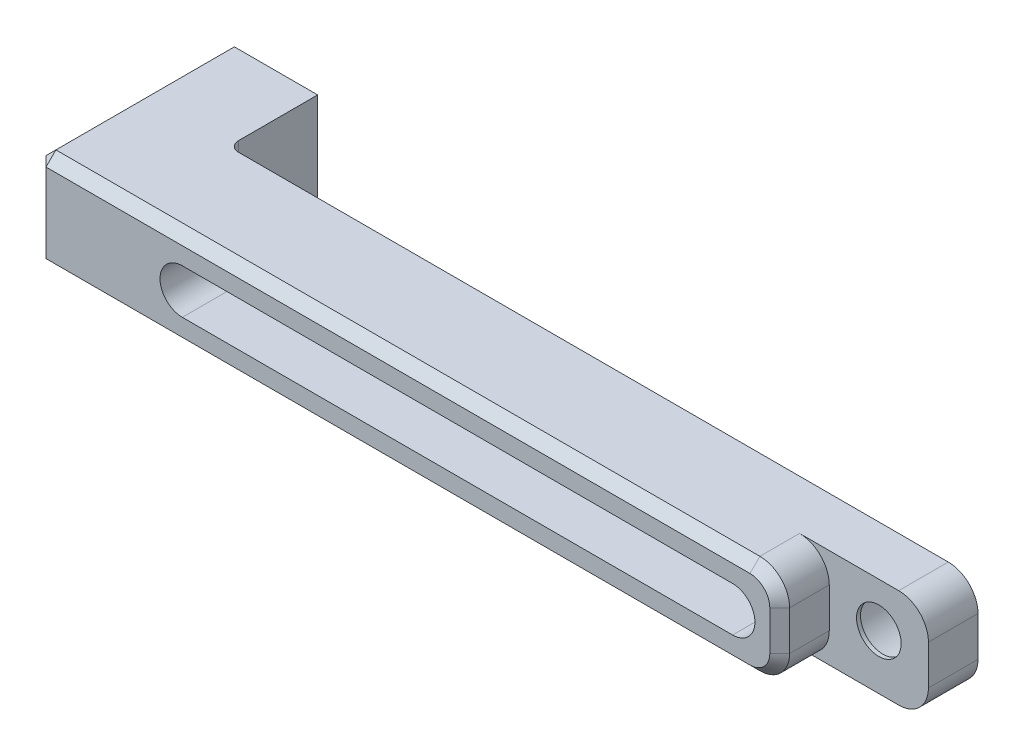
from build123d import *

# Parameters (mm, degrees)
SKETCH1_W                                            = 85
SKETCH1_H                                            = 10
BOSS_EXTRUDE1_DEPTH                                  = 10
CUT_EXTRUDE1_DEPTH                                   = 4.4
CUT_EXTRUDE2_DEPTH                                   = 45.018291652
SKETCH4_W                                            = 9.4
SKETCH4_H                                            = 10
BOSS_EXTRUDE2_DEPTH                                  = 10
SKETCH5_W                                            = 10
SKETCH5_H                                            = 10
CUT_EXTRUDE3_DEPTH                                   = 5
M6_TAPPED_HOLE1_D                                    = 5
M6_TAPPED_HOLE1_DEPTH                                = 5
M6_TAPPED_HOLE1_TIP                                  = 1.502151548
CBORE_FOR_M4_HEXAGON_SOCKET_HEAD_CAP_SCR_D           = 4.5
CBORE_FOR_M4_HEXAGON_SOCKET_HEAD_CAP_SCR_DEPTH       = 14
CBORE_FOR_M4_HEXAGON_SOCKET_HEAD_CAP_SCR_CBORE_D     = 8
CBORE_FOR_M4_HEXAGON_SOCKET_HEAD_CAP_SCR_CBORE_DEPTH = 4.6
CBORE_FOR_M4_HEXAGON_SOCKET_HEAD_CAP_SCR_TIP         = 1.351936393
FILLET1_R                                            = 3
FILLET2_R                                            = 1
CHAMFER1_SIZE                                        = 1


with BuildPart() as part:
    # Sketch1 → Boss-Extrude1 (new body)
    with BuildSketch(Plane(origin=(0, 0, 0), x_dir=(1, 0, 0), z_dir=(0, 1, 0))):
        Rectangle(SKETCH1_W, SKETCH1_H)
    extrude(amount=BOSS_EXTRUDE1_DEPTH)

    # Sketch2 → Cut-Extrude1 (cut)
    with BuildSketch(Plane.XY.offset(-5)):
        with BuildLine():
            Line((-27.75, 9), (27.75, 9))
            ThreePointArc((27.75, 9), (31.75, 5), (27.75, 1))
            Line((27.75, 1), (-27.75, 1))
            ThreePointArc((-27.75, 1), (-31.75, 5), (-27.75, 9))
        make_face()
    extrude(amount=CUT_EXTRUDE1_DEPTH, mode=Mode.SUBTRACT)

    # Sketch3 → Cut-Extrude2 (cut, through all)
    with BuildSketch(Plane(origin=(0, 0, -0.6), x_dir=(-1, 0, 0), z_dir=(0, 0, -1))):
        with BuildLine():
            Line((-27.75, 7.25), (27.75, 7.25))
            ThreePointArc((27.75, 7.25), (30, 5), (27.75, 2.75))
            Line((27.75, 2.75), (-27.75, 2.75))
            ThreePointArc((-27.75, 2.75), (-30, 5), (-27.75, 7.25))
        make_face()
    extrude(amount=-CUT_EXTRUDE2_DEPTH, mode=Mode.SUBTRACT)

    # Sketch4 → Boss-Extrude2 (add)
    with BuildSketch(Plane.XY.offset(-5)):
        with Locations((-37.8, 5)):
            Rectangle(SKETCH4_W, SKETCH4_H)
    extrude(amount=-BOSS_EXTRUDE2_DEPTH)

    # Sketch5 → Cut-Extrude3 (cut)
    with BuildSketch(Plane.XY.offset(5)):
        with Locations((37.5, 5)):
            Rectangle(SKETCH5_W, SKETCH5_H)
    extrude(amount=-CUT_EXTRUDE3_DEPTH, mode=Mode.SUBTRACT)

    # M6 Tapped Hole1
    with Locations(Plane(origin=(0, 0, -15), x_dir=(-1, 0, 0), z_dir=(0, 0, -1))):
        with Locations((37.8, 4.802472567)):
            Hole(M6_TAPPED_HOLE1_D / 2, depth=M6_TAPPED_HOLE1_DEPTH)
            with Locations((0, 0, -(M6_TAPPED_HOLE1_DEPTH + M6_TAPPED_HOLE1_TIP / 2))):  # 118° drill point
                Cone(0, M6_TAPPED_HOLE1_D / 2, M6_TAPPED_HOLE1_TIP, mode=Mode.SUBTRACT)

    # CBORE for M4 Hexagon socket head cap screws1
    with Locations(Plane(origin=(0, 0, -5), x_dir=(-1, 0, 0), z_dir=(0, 0, -1))):
        with Locations((-37.5, 5.5)):
            CounterBoreHole(CBORE_FOR_M4_HEXAGON_SOCKET_HEAD_CAP_SCR_D / 2, CBORE_FOR_M4_HEXAGON_SOCKET_HEAD_CAP_SCR_CBORE_D / 2, CBORE_FOR_M4_HEXAGON_SOCKET_HEAD_CAP_SCR_CBORE_DEPTH, depth=CBORE_FOR_M4_HEXAGON_SOCKET_HEAD_CAP_SCR_DEPTH)
            with Locations((0, 0, -(CBORE_FOR_M4_HEXAGON_SOCKET_HEAD_CAP_SCR_DEPTH + CBORE_FOR_M4_HEXAGON_SOCKET_HEAD_CAP_SCR_TIP / 2))):  # 118° drill point
                Cone(0, CBORE_FOR_M4_HEXAGON_SOCKET_HEAD_CAP_SCR_D / 2, CBORE_FOR_M4_HEXAGON_SOCKET_HEAD_CAP_SCR_TIP, mode=Mode.SUBTRACT)

    # Fillet1
    fillet1_edges = [part.edges().sort_by_distance(p)[0] for p in [
        (42.5, 0, -2.5),
        (42.5, 10, -2.5),
        (32.5, 0, 2.5),
        (32.5, 10, 2.5),
    ]]
    fillet(fillet1_edges, radius=FILLET1_R)

    # Fillet2
    fillet2_edges = [part.edges().sort_by_distance(p)[0] for p in [
        (-33.1, 5, -5),
    ]]
    fillet(fillet2_edges, radius=FILLET2_R)

    # Chamfer1
    chamfer1_edges = [part.edges().sort_by_distance(p)[0] for p in [
        (-37.8, 0, -15),
        (-42.5, 5, -15),
        (-37.8, 10, -15),
        (-33.1, 5, -15),
        (-42.5, 10, -5),
        (-6.5, 0, 5),
        (-42.5, 0, -5),
        (-42.5, 5, 5),
        (-6.5, 10, 5),
        (32.5, 5, 5),
        (31.621320344, 9.121320344, 5),
        (31.621320344, 0.878679656, 5),
    ]]
    chamfer(chamfer1_edges, length=CHAMFER1_SIZE)


solid = part.part
